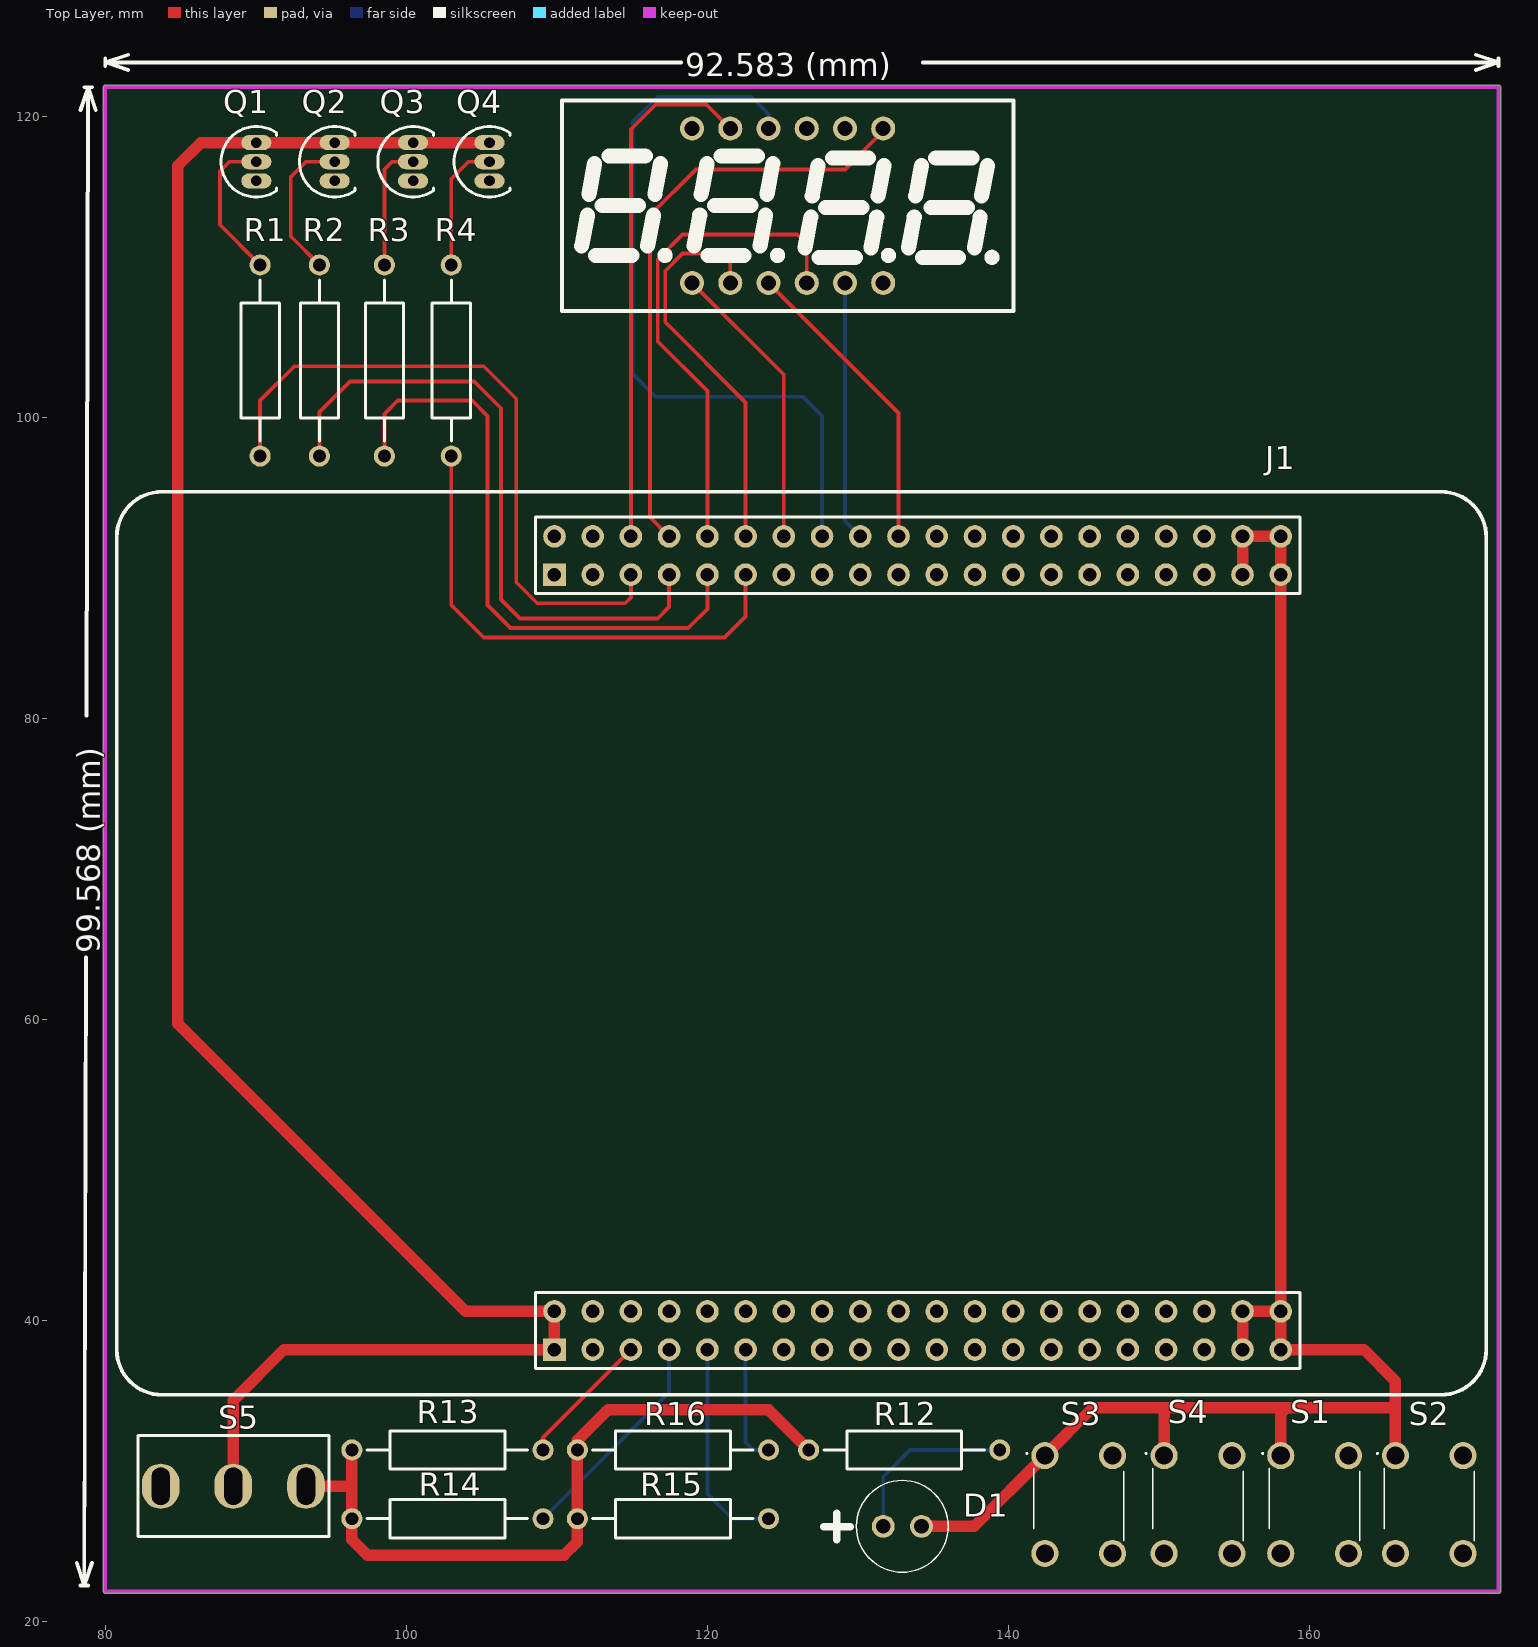
[diagram p0: Top Layer view]
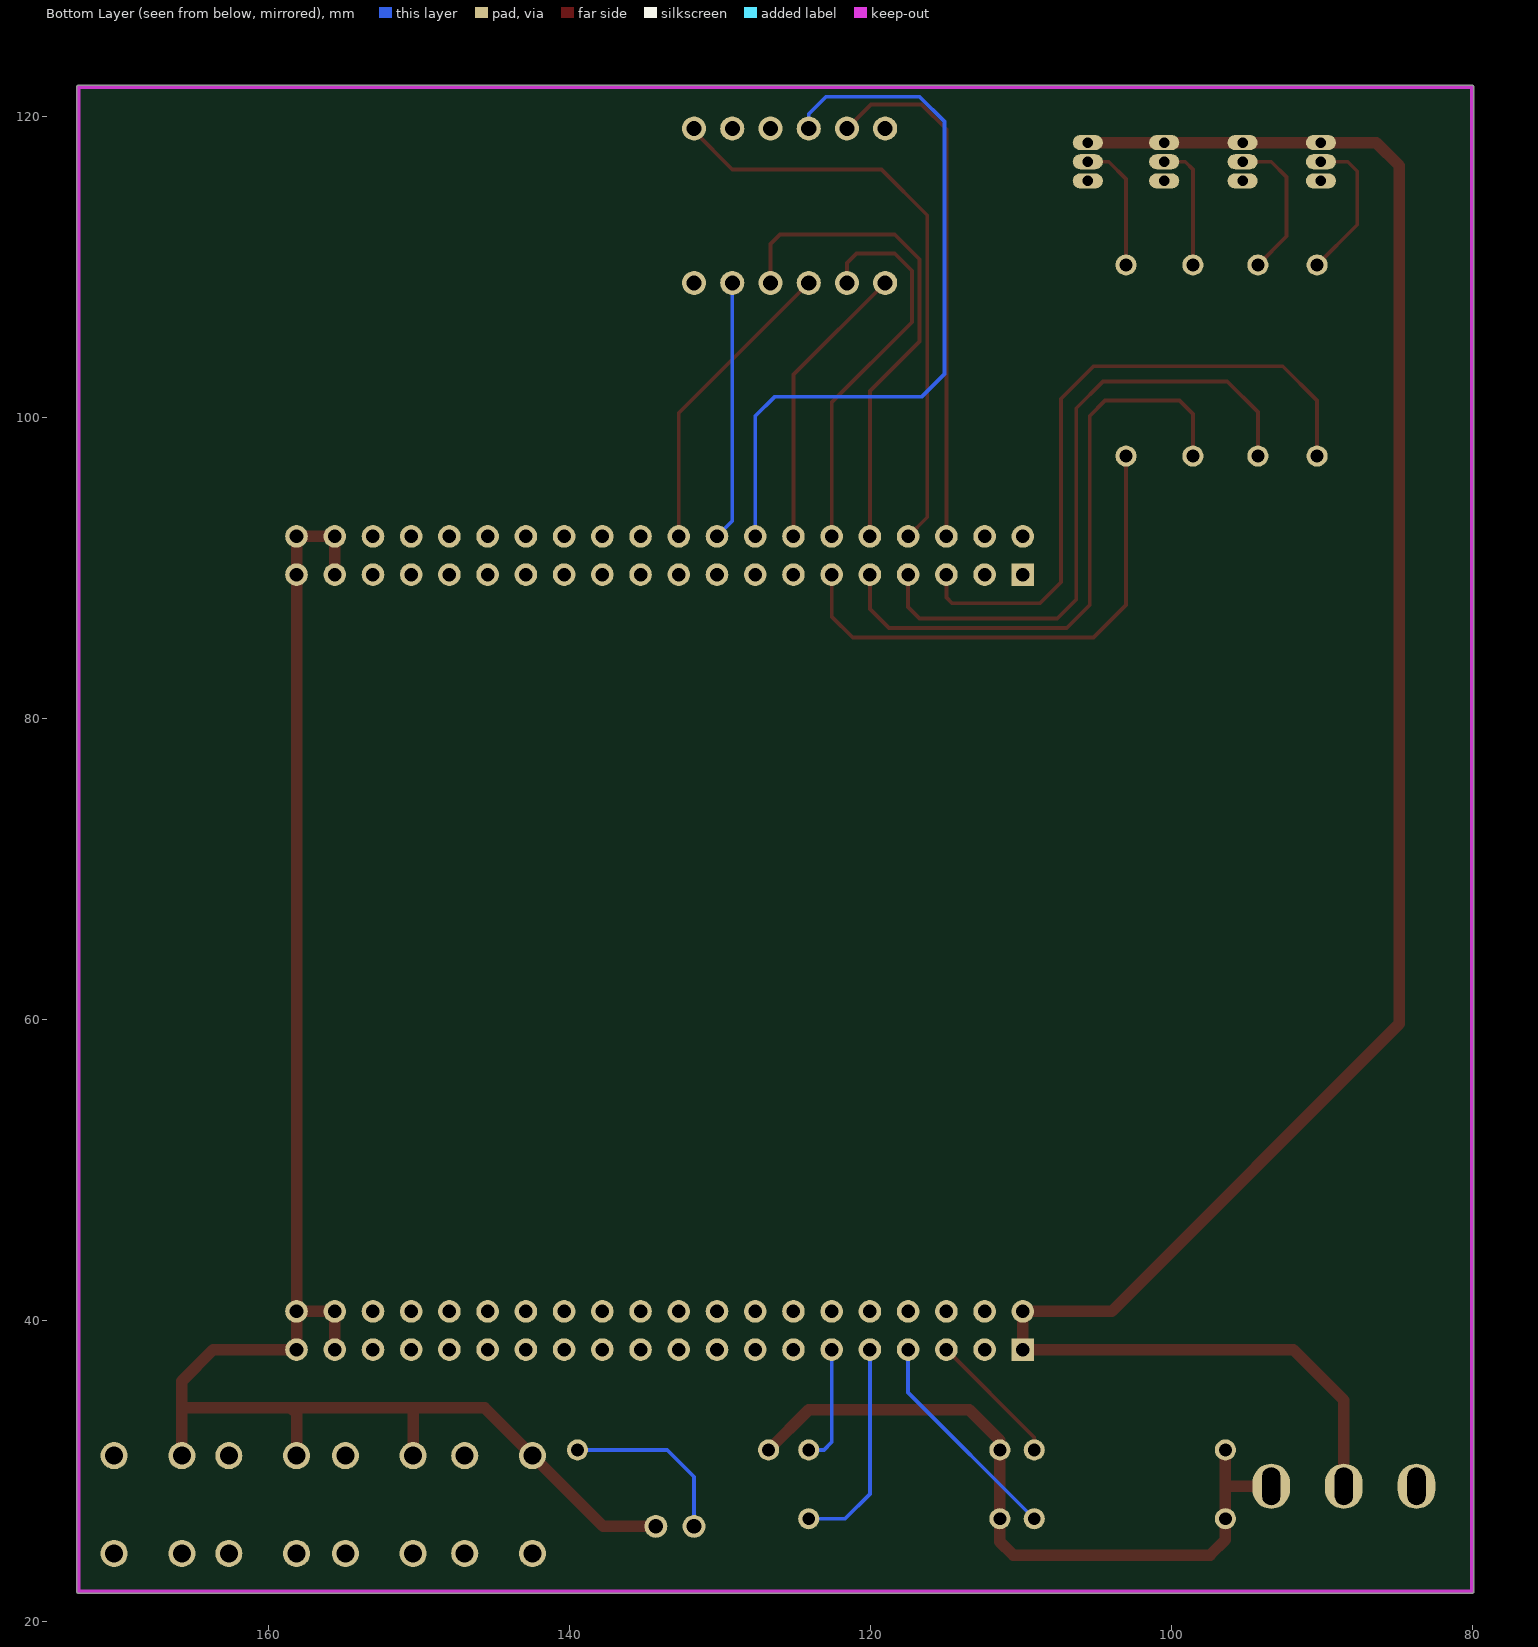
[diagram p1: Bottom Layer view, seen from below]
# Altium PCB MISC89346.PcbDoc
Units mm, origin at the board's own origin, x right, y up, seen from the top; angles counter-clockwise.
Board outline 92.84 x 100.2 mm, 2 copper layers (Top Layer, Bottom Layer); 21 components, 28 nets, 143 pads, 0 vias.

## Layer stack, top to bottom (the 12.6 mil dielectric is the usual default, probably not edited)
Top Solder: solder mask 0.0102, Solder Resist, Dk 3.5
Top Layer: signal copper 0.0356
Dielectric 1: dielectric 0.32, FR-4, Dk 4.8
Bottom Layer: signal copper 0.0356
Bottom Solder: solder mask 0.0102, Solder Resist, Dk 3.5

## Board outline
79.883,21.971 ccw(c80.01,21.971) 80.01,21.844 172.593,21.844 ccw(c172.593,21.971) 172.72,21.971 172.72,121.92 ccw(c172.593,121.92) 172.593,122.047 80.01,122.047 ccw(c80.01,121.92) 79.883,121.92

## Design rules (kind name [scope] priority, off if disabled: settings)
Clearance [All] p1: gap=0.254
MinimumSolderMaskSliver [All] p1: minsoldermaskwidth=0
PolygonConnect [All] p1: connectstyle=Relief reliefconductorwidth=0.254 reliefentries=4 polygonreliefangle="90 Angle" airgapwidth=0.254
RoutingVias [All] p1: holewidth=0.711 width=1.27 viastyle="Through Hole" minholewidth=0.711 minwidth=1.27 maxholewidth=0.711 maxwidth=1.27
SilkToSilkClearance [All] p1: silktosilkclearance=0
SilkToSolderMaskClearance [IsPad] p1: minsilkscreentomaskgap=0 clearancetoexposedcopper=TRUE
SolderMaskExpansion [All] p1: expansion=0.102
Width [All] p1: maxlimit=0.762 minlimit=0.254 preferedwidth=0.254
27 further rules are at their usual default settings.

## Components (designator, comment, footprint, x,y, rotation, side; value= is the part's Value field where it differs from the comment)
D1 "LED0" LED_TH_HLMP4700 131.699,26.289 r0 top
J1 "COREBOARD_CONNECTOR" coreboard_connector 109.855,38.035 r0 top
Q1 "PNP" TO-92 90.043,116.967 r0 top
Q2 "PNP" TO-92 95.25,116.967 r0 top
Q3 "PNP" TO-92 100.457,116.967 r0 top
Q4 "PNP" TO-92 105.537,116.967 r0 top
R1 "" AXIAL-0.5 90.297,103.759 r90 top
R2 "" AXIAL-0.5 94.234,103.759 r90 top
R3 "" AXIAL-0.5 98.552,103.759 r90 top
R4 "" AXIAL-0.5 102.997,103.759 r90 top
R12 "Res2" AXIAL-0.5 133.096,31.369 r180 top
R13 "Res2" AXIAL-0.5 102.743,31.369 r180 top
R14 "Res2" AXIAL-0.5 102.743,26.797 r180 top
R15 "Res2" AXIAL-0.5 117.729,26.797 r180 top
R16 "Res2" AXIAL-0.5 117.729,31.369 r180 top
S1 "SW-PB" TS665CJ 158.115,30.988 r0 top
S2 "SW-PB" TS665CJ 165.735,30.988 r0 top
S3 "SW-PB" TS665CJ 142.439,30.988 r0 top
S4 "SW-PB" TS665CJ 150.368,30.988 r0 top
S5 "SW-SPST" SS12D10 93.345,28.956 r180 top
? "DIG-4" DIG-4 125.857,113.157 r0 top

## Footprints (in the part's own frame and the unit in brackets; to place one, negate y for a bottom-side part, rotate by r counter-clockwise, add the part's x,y. Pads: shape width x height; smd on the part's side, far side on the other; paste and mask are expansions set on the pad)
AXIAL-0.5 [mm] "Axial Device, Thru-Hole; 2 Leads; 0.5 in Pin Spacing"
  round 1.4 hole 0.85: 1(-6.35,0) 2(6.35,0)
  silkscreen extent -5.33,-1.27 5.33,1.27
coreboard_connector [mm] "Connector; Header40; 20x2 Position"
  rect 1.5x1.5 hole 0.9: 1(0,0) 41(0,51.5)
  round 1.5 hole 0.9: 2(0,2.54) 3(2.54,0) 4(2.54,2.54) 5(5.08,0) 6(5.08,2.54) 7(7.62,0) 8(7.62,2.54) 9(10.16,0) 10(10.16,2.54) 11(12.7,0) 12(12.7,2.54) 13(15.24,0) 14(15.24,2.54) 15(17.78,0) 16(17.78,2.54) 17(20.32,0) 18(20.32,2.54) 19(22.86,0) 20(22.86,2.54) 21(25.4,0) 22(25.4,2.54) 23(27.94,0) 24(27.94,2.54) 25(30.48,0) 26(30.48,2.54) 27(33.02,0) 28(33.02,2.54) 29(35.56,0) 30(35.56,2.54) 31(38.1,0) 32(38.1,2.54) 33(40.64,0) 34(40.64,2.54) 35(43.18,0) 36(43.18,2.54) 37(45.72,0) 38(45.72,2.54) 39(48.26,0) 40(48.26,2.54) 42(0,54.04) 43(2.54,51.5) 44(2.54,54.04) 45(5.08,51.5) 46(5.08,54.04) 47(7.62,51.5) 48(7.62,54.04) 49(10.16,51.5) 50(10.16,54.04) 51(12.7,51.5) 52(12.7,54.04) 53(15.24,51.5) 54(15.24,54.04) 55(17.78,51.5) 56(17.78,54.04) 57(20.32,51.5) 58(20.32,54.04) 59(22.86,51.5) 60(22.86,54.04) 61(25.4,51.5) 62(25.4,54.04) 63(27.94,51.5) 64(27.94,54.04) 65(30.48,51.5) 66(30.48,54.04) 67(33.02,51.5) 68(33.02,54.04) 69(35.56,51.5) 70(35.56,54.04) 71(38.1,51.5) 72(38.1,54.04) 73(40.64,51.5) 74(40.64,54.04) 75(43.18,51.5) 76(43.18,54.04) 77(45.72,51.5) 78(45.72,54.04) 79(48.26,51.5) 80(48.26,54.04)
  silkscreen extent -29.09,-3 61.91,57, body extent -1.27,-1.27 49.53,55.31, height 7.58
DIG-4 [mm]
  round 1.6 hole 1 mask+0.051: 1(-6.858,-4.241) 2(-4.318,-4.241) 3(-1.778,-4.241) 4(0.762,-4.241) 5(3.302,-4.241) 6(5.842,-4.241) 7(5.842,6.019) 8(3.302,6.019) 9(0.762,6.019) 10(-1.778,6.019) 11(-4.318,6.019) 12(-6.858,6.019)
  silkscreen extent -15.51,-6.11 14.49,7.89
LED_TH_HLMP4700 [mm]
  round 1.521 hole 0.978: 1(0,0) 2(2.54,0)
  silkscreen extent -3.94,-3.05 4.32,3.05, body extent -1.66,-2.9 4.14,2.9, height 9.6
SS12D10 [mm]
  oval 2.5x3 hole 1.2 slot 2.5 at 90 deg: 1(4.826,0) 2(0,0) 3(9.652,0)
  silkscreen extent -1.52,-3.38 11.18,3.35, body extent -1.67,-3.43 11.33,3.37, height 9.4
TO-92 [mm]
  oval 2x1 hole 0.7: 1(0,-1.27) 2(0,0) 3(0,1.27)
  silkscreen extent -2.34,-2.34 1.35,2.34
TS665CJ [mm]
  round 1.8 hole 1.2: A1(0,0) B1(4.5,0) C1(0,-6.5) D1(4.5,-6.5)
  silkscreen extent -1.25,-5.65 5.25,0.2, body extent -0.75,-6.9 5.25,0.4, height 5.25

## Part data
D1: "Typical INFRARED GaAs LED"
Q1 Q2 Q3 Q4: "PNP Bipolar Transistor"
R1 R2 R3 R4: library part Res2, "Resistor"
R12 R13 R14 R15 R16: "Resistor"
S1 S2 S3 S4: "Switch"
S5: "Single-Pole, Single-Throw Switch"

## Nets (pads, with @x,y where several pads share a name; then routed paths per layer and width w, separated by ;. In a path a pad name is that pad's centre, name@x,y a point inside that pad or via, vN(x,y) a via of type N, cw(c..) or ccw(c..) an arc to the next point about the centre after c; other vN are vias at no path point)
A: ?.11 J1.46 | length 35
  Top Layer w0.254: J1.46 114.935,119.126 116.586,120.777 119.938,120.777 ?.11
B: ?.7 J1.48 | length 39.8
  Top Layer w0.254: J1.48 116.205,93.345 116.205,113.411 119.253,116.459 129.159,116.459 131.699,118.999 ?.7
C: ?.4 J1.50 | length 33.2
  Top Layer w0.254: J1.50 120.015,101.727 116.713,105.029 116.713,110.49 118.364,112.141 125.984,112.141 126.619,111.506 ?.4
D: ?.2 J1.52 | length 26.2
  Top Layer w0.254: ?.2 121.539,110.236 120.904,110.871 118.364,110.871 117.221,109.728 117.221,106.299 122.555,100.965 J1.52
DIG1: ?.12
DIG2: ?.9
DIG3: ?.8
DIG4: ?.6
DP: ?.3 J1.60 | length 20.4
  Top Layer w0.254: ?.3 132.715,100.28 J1.60
E: ?.1 J1.54 | length 19.4
  Top Layer w0.254: ?.1 125.095,102.82 J1.54
F: ?.10 J1.56 | length 49.6
  Bottom Layer w0.254: ?.10 124.079,120.142 122.936,121.285 116.713,121.285 115.062,119.634 115.062,102.87 116.586,101.346 126.365,101.346 127.635,100.076 J1.56
G: ?.5 J1.58 | length 17.3
  Bottom Layer w0.254: ?.5 129.159,93.091 J1.58
GND: D1.2 J1.37 J1.38 J1.39 J1.40 J1.77 J1.78 J1.79 J1.80 S1.A1 S2.A1 S3.A1 S4.A1 | length 119
  Top Layer w0.762: D1.2 137.74,26.289 S3.A1 145.614,34.163 150.368,34.163 ; S4.A1 150.368,34.163 ; J1.37 J1.38 J1.40 ; J1.77 J1.78 J1.80 J1.79 J1.40 ; S1.A1 158.115,33.782 158.496,34.163 ; S2.A1 165.735,34.036 ; 150.368,34.163 158.496,34.163 ; J1.40 J1.39 163.641,38.035 165.735,35.941 165.735,34.036 ; 158.496,34.163 165.608,34.163 165.735,34.036
NetD1_1: D1.1 R12.1 | length 11.8
  Bottom Layer w0.254: D1.1 131.699,29.591 133.477,31.369 R12.1
NetQ1_2: Q1.2 R1.2 | length 10
  Top Layer w0.254: Q1.2 88.265,116.967 87.63,116.332 87.63,112.776 R1.2
NetQ2_2: Q2.2 R2.2 | length 10
  Top Layer w0.254: R2.2 92.329,112.014 92.329,115.951 93.345,116.967 Q2.2
NetQ3_2: Q3.2 R3.2 | length 8.5
  Top Layer w0.254: R3.2 98.552,116.459 99.06,116.967 Q3.2
NetQ4_2: Q4.2 R4.2 | length 8.7
  Top Layer w0.254: R4.2 102.997,115.824 104.14,116.967 Q4.2
NetR12_2: R12.2 R13.2 R14.2 R15.2 R16.2 S5.2 | length 48.8
  Top Layer w0.762: S5.2 96.393,28.956 ; R13.2 96.393,28.956 ; R12.2 124.079,34.036 113.411,34.036 111.379,32.004 R16.2 R15.2 111.379,25.273 110.49,24.384 97.409,24.384 96.393,25.4 R14.2 96.393,28.956
VCC: J1.1 J1.2 Q1.3 Q2.3 Q3.3 Q4.3 S5.1 | length 142.3
  Top Layer w0.762: S5.1 88.519,34.671 91.883,38.035 J1.1 J1.2 103.951,40.575 84.836,59.69 84.836,116.713 86.36,118.237 Q1.3 Q2.3 Q3.3 Q4.3
W1: J1.5 R13.1 | length 9.1
  Top Layer w0.254: R13.1 109.093,32.193 J1.5
W2: J1.7 R14.1 | length 15.1
  Top Layer w0.254: J1.7@117.221,37.781 J1.7
  Bottom Layer w0.254: R14.1 117.475,35.179 J1.7
W3: J1.9 R15.1 | length 14.3
  Bottom Layer w0.254: J1.9 120.015,28.448 121.666,26.797 R15.1
W4: J1.11 R16.1 | length 7.9
  Bottom Layer w0.254: J1.11 122.555,31.877 123.063,31.369 R16.1
W5: J1.45 R1.1 | length 44.6
  Top Layer w0.254: R1.1 90.297,101.092 92.583,103.378 105.156,103.378 107.315,101.219 107.315,89.027 108.712,87.63 114.554,87.63 114.935,88.011 J1.45
W6: J1.47 R2.1 | length 43.4
  Top Layer w0.254: R2.1 94.234,100.33 96.266,102.362 104.521,102.362 106.299,100.584 106.299,87.884 107.569,86.614 116.713,86.614 117.475,87.376 J1.47
W7: J1.49 R3.1 | length 41.1
  Top Layer w0.254: R3.1 98.552,100.203 99.441,101.092 104.394,101.092 105.41,100.076 105.41,87.503 106.934,85.979 118.745,85.979 120.015,87.249 J1.49
W8: J1.51 R4.1 | length 33.7
  Top Layer w0.254: R4.1 102.997,87.503 105.156,85.344 121.158,85.344 122.555,86.741 J1.51
pads on no net: J1.3 J1.4 J1.6 J1.8 J1.10 J1.12 J1.13 J1.14 J1.15 J1.16 J1.17 J1.18 J1.19 J1.20 J1.21 J1.22 J1.23 J1.24 J1.25 J1.26 J1.27 J1.28 J1.29 J1.30 J1.31 J1.32 J1.33 J1.34 J1.35 J1.36 J1.41 J1.42 J1.43 J1.44 J1.53 J1.55 J1.57 J1.59 J1.61 J1.62 J1.63 J1.64 J1.65 J1.66 J1.67 J1.68 J1.69 J1.70 J1.71 J1.72 J1.73 J1.74 J1.75 J1.76 Q1.1 Q2.1 Q3.1 Q4.1 S1.B1 S1.C1 S1.D1 S2.B1 S2.C1 S2.D1 S3.B1 S3.C1 S3.D1 S4.B1 S4.C1 S4.D1 S5.3

## Keep-outs
Keep-Out Layer:
  lines w0.254: 172.593,117.856 172.593,121.92 111.76,121.92 80.01,121.92 80.01,21.971 172.593,21.971 172.593,118.237

## Silkscreen, mask and mechanical layers (free items; w line width, h text height)
Top Overlay:
  lines w0.254: 78.109,23.877 78.613,22.352 ; 78.355,120.397 78.867,121.92 ; 78.359,22.353 78.867,22.351 ; 78.613,121.921 79.121,121.919 ; 78.72,64.112 78.613,22.352 ; 78.76,80.16 78.867,121.92 ; 79.125,23.875 78.613,22.352 ; 79.371,120.395 78.867,121.92 ; 80.01,123.317 80.01,123.825 ; 81.534,123.063 80.01,123.571 ; 81.534,124.079 80.01,123.571 ; 118.278,123.571 80.01,123.571 ; 134.325,123.571 172.593,123.571 ; 171.069,123.063 172.593,123.571 ; 171.069,124.079 172.593,123.571 ; 172.593,123.317 172.593,123.825
  text "92.583 (mm)" at 118.532,122.657 h1.52
  text "99.568 (mm)" at 79.634,64.364 h1.52 r89.85